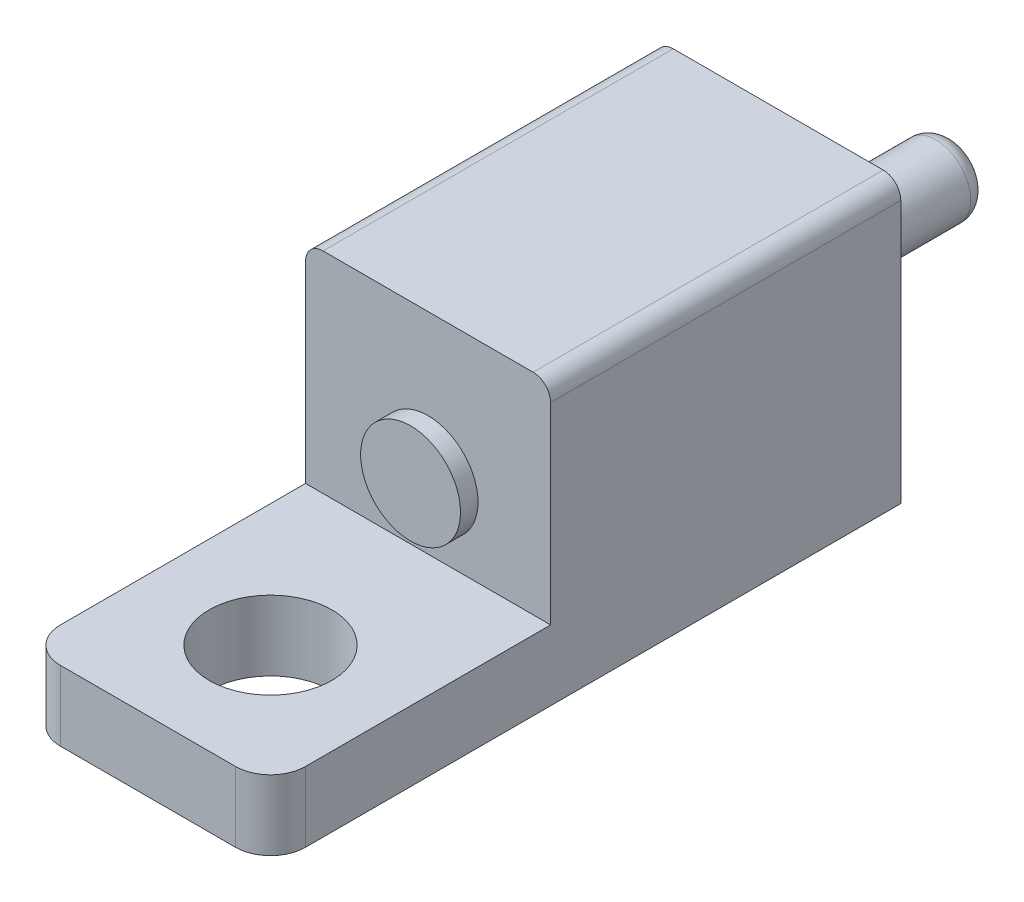
SolidWorks part; units mm, degrees
ref_plane "Front Plane" through (0, 0, 0) normal (0, 0, 1) x (1, 0, 0)
ref_plane "Top Plane" through (0, 0, 0) normal (0, 1, 0) x (1, 0, 0)
ref_plane "Right Plane" through (0, 0, 0) normal (1, 0, 0) x (0, 0, -1)
other "Configuration Table"
sketch "Sketch1" plane through (0, 0, 0) normal (0, 0, 1) x (1, 0, 0)
  line L1 (-3.5, 4) -> (3.5, 4)
  line L2 (-3.5, 4) -> (-3.5, -4)
  line L3 (-3.5, -4) -> (3.5, -4)
  line L4 (3.5, 4) -> (3.5, -4)
  line L5 (-3.5, 4) -> (3.5, -4) construction
  line L6 (-3.5, -4) -> (3.5, 4) construction
  point P0 (0, 0)
  dimension "D1" = 7
  dimension "D2" = 8
extrude "Boss-Extrude1" add sketch "Sketch1" along normal blind 10
sketch "Sketch2" plane through (0, 0, 10) normal (0, 0, 1) x (1, 0, 0)
  line L1 (-3.5, -2) -> (3.5, -2)
  line L2 (-3.5, -2) -> (-3.5, -4)
  line L3 (-3.5, -4) -> (3.5, -4)
  line L4 (3.5, -2) -> (3.5, -4)
  line L5 (-3.5, -2) -> (3.5, -4) construction
  line L6 (-3.5, -4) -> (3.5, -2) construction
  point P0 (0, -3)
  dimension "D1" = 2
  dimension "D2" = 7
extrude "Boss-Extrude2" add sketch "Sketch2" along normal blind 8
sketch "Sketch3" plane through (0, 0, 0) normal (0, 0, -1) x (-1, 0, 0)
  circle A0 centre (0, 0) radius 1
  dimension "D1" = 2
extrude "Boss-Extrude3" add sketch "Sketch3" along normal blind 5
fillet "Fillet1" radius 0.5 1 edges at (-1, 0, -5)
sketch "Sketch4" plane through (0, 0, 0) normal (0, 0, -1) x (-1, 0, 0)
  circle A0 centre (0, 0) radius 1.4902
extrude "Boss-Extrude4" add sketch "Sketch4" along normal blind 1
sketch "Sketch5" plane through (0, 0, 10) normal (0, 0, 1) x (1, 0, 0)
  circle A0 centre (0, 0) radius 1.4267
extrude "Boss-Extrude5" add sketch "Sketch5" along normal blind 0.5
fillet "Fillet3" radius 0.5 2 edges at (-3.5, 4, 5) (3.5, 4, 5)
fillet "Fillet4" radius 1 2 edges at (-3.5, -3, 18) (3.5, -3, 18)
sketch "Sketch6" plane through (0, -2, 0) normal (0, 1, 0) x (1, 0, 0)
  line L0 (2.5, -18) -> (-2.5, -18) construction
  circle A0 centre (0, -14.5) radius 1.75
  dimension "D1" = 3.5
  dimension "D2" = 3.5
extrude "Cut-Extrude1" cut sketch "Sketch6" against normal through all
